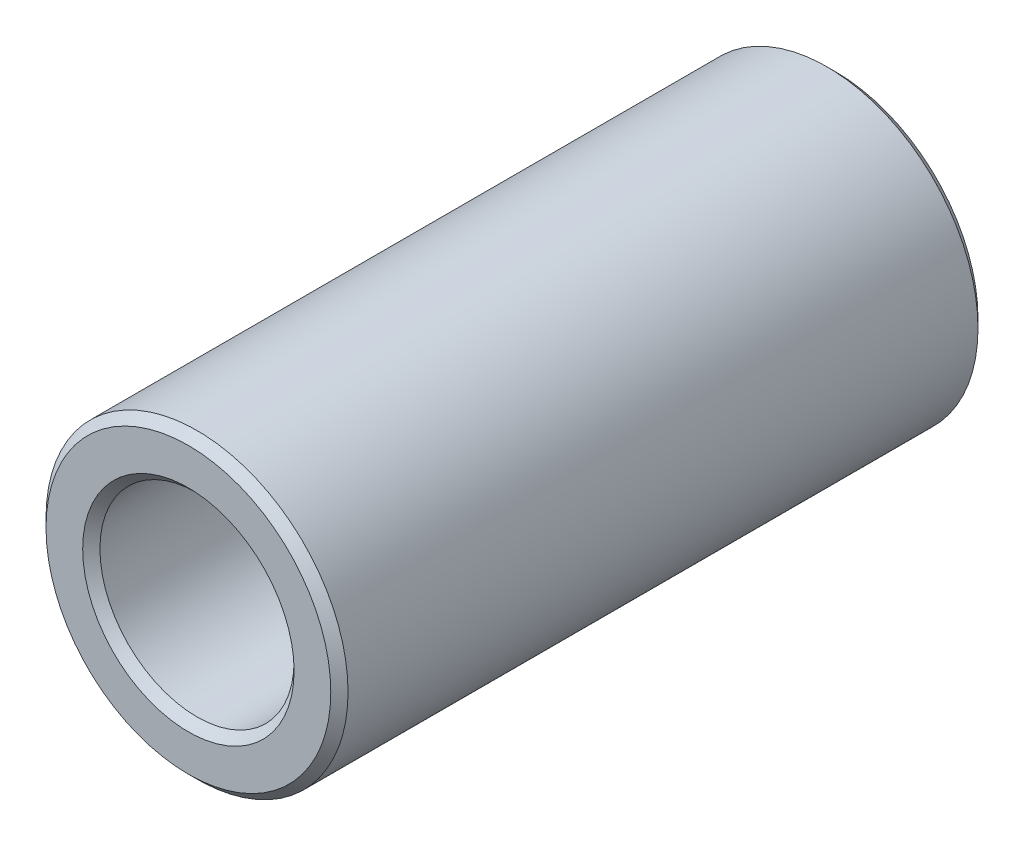
SolidWorks part; units mm, degrees
material "尼龙 101"
ref_plane "Front Plane" through (0, 0, 0) normal (0, 0, 1) x (1, 0, 0)
ref_plane "Top Plane" through (0, 0, 0) normal (0, 1, 0) x (1, 0, 0)
ref_plane "Right Plane" through (0, 0, 0) normal (1, 0, 0) x (0, 0, -1)
sketch "Sketch1" plane through (0, 0, 0) normal (0, 0, 1) x (1, 0, 0)
  circle A0 centre (0, 0) radius 3.5
  circle A1 centre (0, 0) radius 2.25
  dimension "D1" = 7
  dimension "D2" = 4.5
extrude "Boss-Extrude1" add sketch "Sketch1" along normal mid plane 15
chamfer "Chamfer1" distance 0.2 angle 45 4 edges at (2.25, 0, -7.5) (3.5, 0, -7.5) (2.25, 0, 7.5) (3.5, 0, 7.5)
